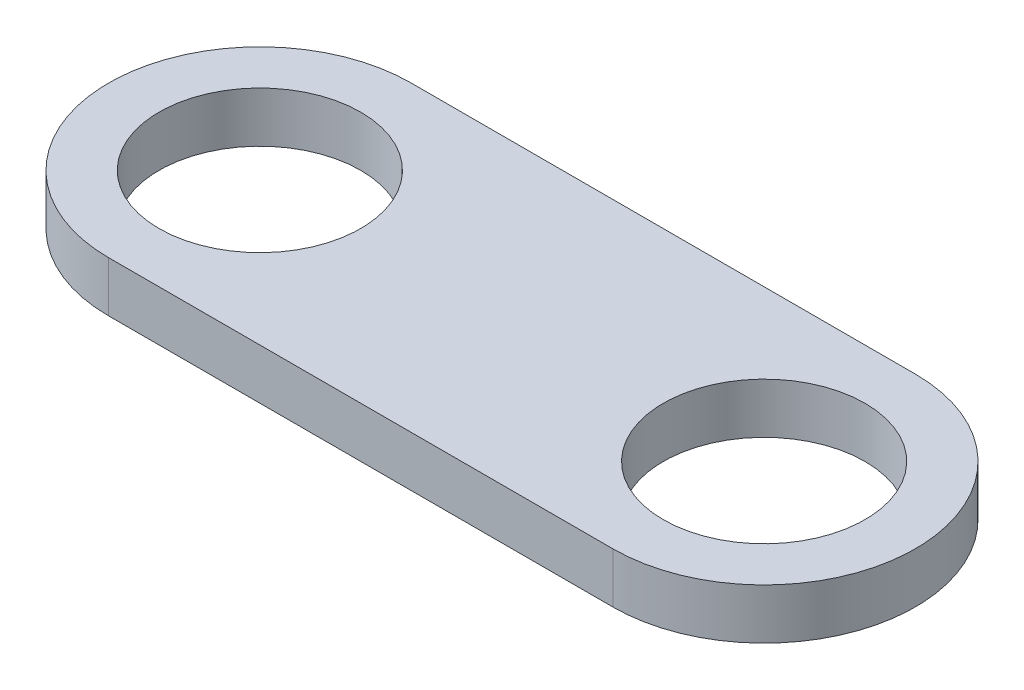
SolidWorks part; units mm, degrees
material "合金钢"
ref_plane "前视基准面" through (0, 0, 0) normal (0, 0, 1) x (1, 0, 0)
ref_plane "上视基准面" through (0, 0, 0) normal (0, 1, 0) x (1, 0, 0)
ref_plane "右视基准面" through (0, 0, 0) normal (1, 0, 0) x (0, 0, -1)
sketch "草图1" plane through (0, 0, 0) normal (0, 1, 0) x (1, 0, 0)
  line L0 (-50, 0) -> (50, 0) construction
  line L1 (-50, 30) -> (50, 30)
  line L2 (-50, -30) -> (50, -30)
  arc A0 (-50, 30) -> (-50, -30) centre (-50, 0) ccw
  arc A1 (50, -30) -> (50, 30) centre (50, 0) ccw
  circle A2 centre (50, 0) radius 20
  circle A3 centre (-50, 0) radius 20
  point P2 (0, 0)
  dimension "D1" = 30
  dimension "D3" = 40
  dimension "D2" = 100
extrude "凸台-拉伸1" add sketch "草图1" along normal blind 10
